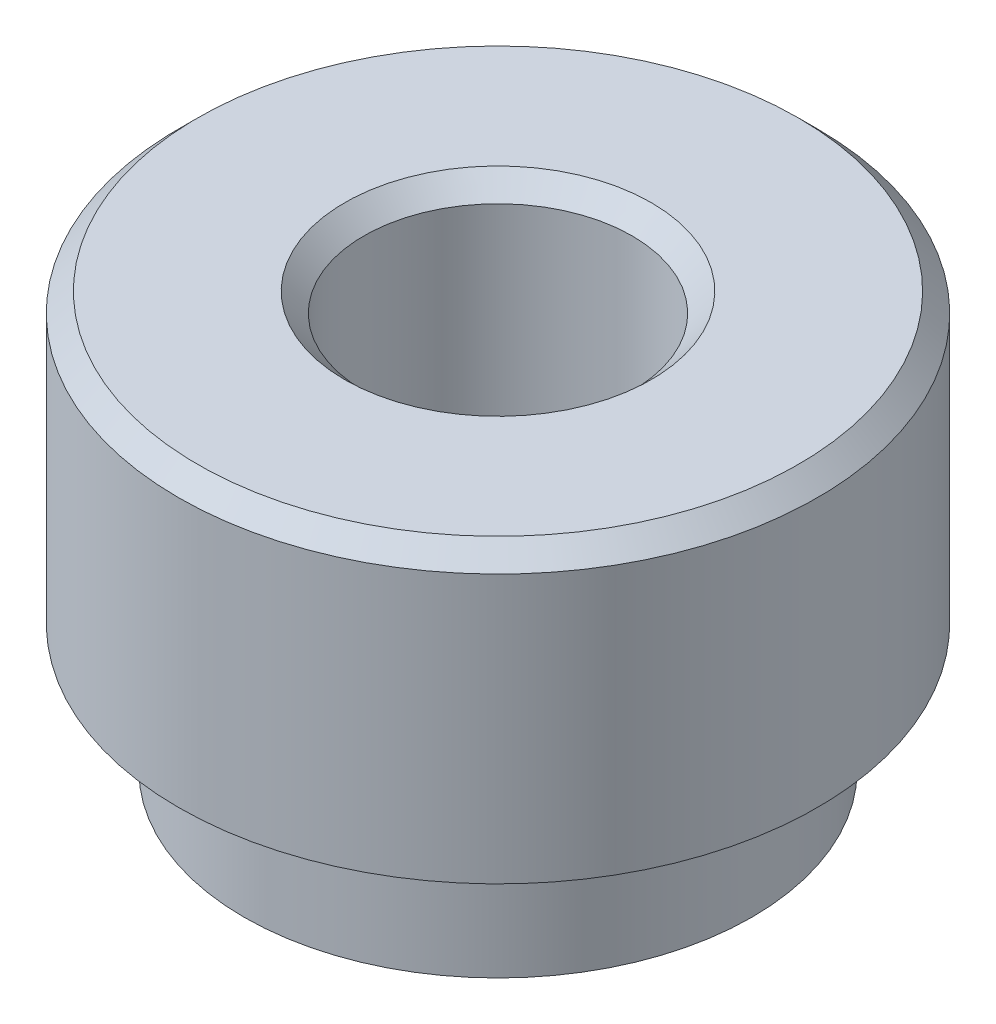
from build123d import *

# Parameters (mm, degrees)
HOLE_WIZARD_M5_1_D = 4.2
CHAMFER_1_SIZE     = 0.3


with BuildPart() as part:
    # 草图1 → 旋转1 (revolve)
    with BuildSketch(Plane.XY, mode=Mode.PRIVATE) as revolve_1_sk:
        Polygon((0, 6.5), (-5, 6.5), (-5, 2), (-3.975, 2), (-3.975, 0), (-3.25, 0), (-3.25, 2), (0, 2), align=None)
    revolve(revolve_1_sk.sketch.rotate(Axis((0, 0, 0), (0, 1, 0)), 270), axis=Axis((0, 0, 0), (0, 1, 0)))

    # M5 螺纹孔1 (through all)
    with Locations(Plane(origin=(0, 6.5, 0), x_dir=(1, 0, 0), z_dir=(0, 1, 0))):
        with Locations((0, 0)):
            Hole(HOLE_WIZARD_M5_1_D / 2)

    # 倒角1
    chamfer_1_edges = [part.edges().sort_by_distance(p)[0] for p in [
        (2.1, 2, 0),
        (2.1, 6.5, 0),
        (0, 6.5, 5),
    ]]
    chamfer(chamfer_1_edges, length=CHAMFER_1_SIZE)


solid = part.part
